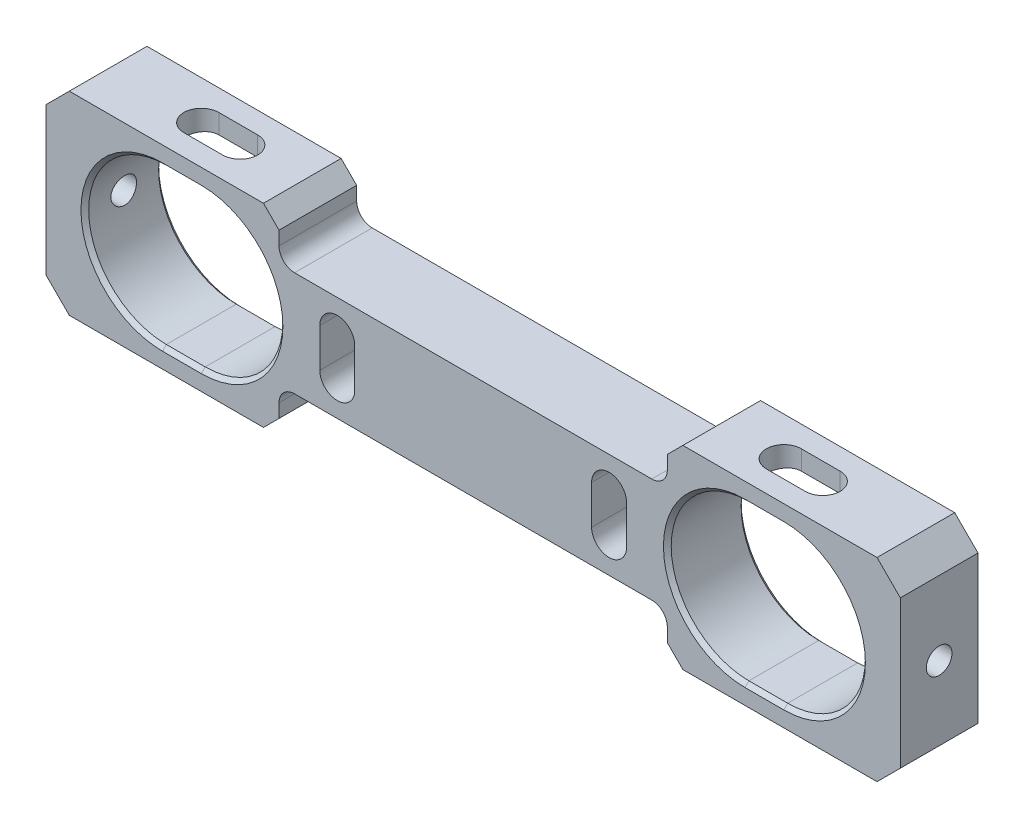
SolidWorks part; units mm, degrees
material "A6061"
ref_plane "Front Plane" through (0, 0, 0) normal (0, 0, 1) x (1, 0, 0)
ref_plane "Top Plane" through (0, 0, 0) normal (0, 1, 0) x (1, 0, 0)
ref_plane "Right Plane" through (0, 0, 0) normal (1, 0, 0) x (0, 0, -1)
sketch "Sketch1" plane through (0, 0, 0) normal (0, 0, 1) x (1, 0, 0)
  line L1 (-55, -12.5) -> (55, -12.5)
  line L2 (-55, -12.5) -> (-55, 12.5)
  line L3 (-55, 12.5) -> (55, 12.5)
  line L4 (55, -12.5) -> (55, 12.5)
  line L5 (-55, -12.5) -> (55, 12.5) construction
  line L6 (-55, 12.5) -> (55, -12.5) construction
  point P0 (0, 0)
  dimension "D1" = 25
  dimension "D2" = 110
extrude "Boss-Extrude1" add sketch "Sketch1" along normal mid plane 10
sketch "Sketch2" plane through (0, 0, 5) normal (0, 0, 1) x (1, 0, 0)
  line L0 (0, 0) -> (0, -23.2819) construction
  line L1 (35, 0) -> (40, 0) construction
  line L2 (35, 10) -> (40, 10)
  line L3 (35, -10) -> (40, -10)
  line L4 (-40, 0) -> (-35, 0) construction
  line L5 (-40, 10) -> (-35, 10)
  line L6 (-40, -10) -> (-35, -10)
  arc A0 (35, 10) -> (35, -10) centre (35, 0) ccw
  arc A1 (40, -10) -> (40, 10) centre (40, 0) ccw
  arc A2 (-40, 10) -> (-40, -10) centre (-40, 0) ccw
  arc A3 (-35, -10) -> (-35, 10) centre (-35, 0) ccw
  point P2 (37.5, 0)
  point P10 (-37.5, 0)
  dimension "D1" = 75
  dimension "D2" = 5
  dimension "D3" = 10
extrude "Cut-Extrude1" cut sketch "Sketch2" against normal through all
chamfer "Chamfer1" distance 3 angle 45 4 edges at (-55, 12.5, 0) (-55, -12.5, 0) (55, -12.5, 0) (55, 12.5, 0)
chamfer "Chamfer2" distance 0.5 angle 45 16 edges at (-50, 0, -5) (-37.5, -10, -5) (-37.5, 10, -5) (-25, 0, -5) (50, 0, -5) (37.5, 10, -5) (37.5, -10, -5) (25, 0, -5) (50, 0, 5) (37.5, 10, 5) (37.5, -10, 5) (25, 0, 5) (-50, 0, 5) (-37.5, -10, 5) (-37.5, 10, 5) (-25, 0, 5)
sketch "Sketch3" plane through (0, 0, 5) normal (0, 0, 1) x (1, 0, 0)
  line L0 (17.5, 2.5) -> (17.5, -2.5) construction
  line L1 (19.75, 2.5) -> (19.75, -2.5)
  line L2 (15.25, 2.5) -> (15.25, -2.5)
  line L3 (-17.5, 2.5) -> (-17.5, -2.5) construction
  line L4 (-15.25, 2.5) -> (-15.25, -2.5)
  line L5 (-19.75, 2.5) -> (-19.75, -2.5)
  line L6 (0, 0) -> (0, -19.6598) construction
  arc A0 (19.75, 2.5) -> (15.25, 2.5) centre (17.5, 2.5) ccw
  arc A1 (15.25, -2.5) -> (19.75, -2.5) centre (17.5, -2.5) ccw
  arc A2 (-15.25, 2.5) -> (-19.75, 2.5) centre (-17.5, 2.5) ccw
  arc A3 (-19.75, -2.5) -> (-15.25, -2.5) centre (-17.5, -2.5) ccw
  point P3 (17.5, 0)
  point P8 (-17.5, 0)
  dimension "D1" = 5
  dimension "D3" = 2.25
  dimension "D2" = 35
extrude "Cut-Extrude2" cut sketch "Sketch3" against normal through all
sketch "Sketch6" plane through (0, 12.5, 0) normal (0, 1, 0) x (1, 0, 0)
  line L0 (-40, 0) -> (-35, 0) construction
  line L1 (-40, 2.25) -> (-35, 2.25)
  line L2 (-40, -2.25) -> (-35, -2.25)
  line L3 (35, 0) -> (40, 0) construction
  line L4 (35, 2.25) -> (40, 2.25)
  line L5 (35, -2.25) -> (40, -2.25)
  line L6 (0, 0) -> (0, -23.5946) construction
  line L7 (-55, -5) -> (-55, 5) construction
  arc A0 (-40, 2.25) -> (-40, -2.25) centre (-40, 0) ccw
  arc A1 (-35, -2.25) -> (-35, 2.25) centre (-35, 0) ccw
  arc A2 (35, 2.25) -> (35, -2.25) centre (35, 0) ccw
  arc A3 (40, -2.25) -> (40, 2.25) centre (40, 0) ccw
  point P3 (-37.5, 0)
  point P8 (37.5, 0)
  dimension "D3" = 2.25
  dimension "D1" = 17.5
  dimension "D2" = 5
extrude "Cut-Extrude3" cut sketch "Sketch6" against normal up to next contours A1 L1 A0 L2
hole_wizard "M4 Tapped Hole1" positions "Sketch8" profile "Sketch7" tap size "M4" standard "ISO"
sketch "Sketch8" plane through (55, 0, 0) normal (1, 0, 0) x (0, 0, -1)
  point P0 (0, 0)
sketch "Sketch7" plane through (55, 0, 0) normal (0, 1, 0) x (0, 0, -1)
  line L0 (0, 0) -> (0, 5)
  line L1 (0, 5) -> (1.65, 5)
  line L2 (1.65, 5) -> (1.65, 0)
  line L5 (1.65, 0) -> (0, 0)
  line L11 (0, -6.35) -> (0, 107.95) construction
  dimension "通孔螺纹孔钻头直径" = 3.3
  dimension "通孔螺纹孔钻头深度" = 5
cosmetic thread "Hole thread1" parameters "D2"=4
hole_wizard "M4 Tapped Hole2" positions "Sketch10" profile "Sketch9" tap size "M4" standard "ISO"
sketch "Sketch10" plane through (-55, 0, 0) normal (-1, 0, 0) x (0, 0, 1)
  point P0 (0, 0)
sketch "Sketch9" plane through (-55, 0, 0) normal (0, 1, 0) x (0, 0, 1)
  line L0 (0, 0) -> (0, 5)
  line L1 (0, 5) -> (1.65, 5)
  line L2 (1.65, 5) -> (1.65, 0)
  line L5 (1.65, 0) -> (0, 0)
  line L11 (0, -6.35) -> (0, 107.95) construction
  dimension "通孔螺纹孔钻头直径" = 3.3
  dimension "通孔螺纹孔钻头深度" = 5
cosmetic thread "Hole thread2" parameters "D2"=4
sketch "Sketch11" plane through (0, 0, -5) normal (0, 0, -1) x (-1, 0, 0)
  line L0 (-17.5, 2.5) -> (-17.5, -2.5) construction
  line L1 (-13.5, 2.5) -> (-13.5, -2.5)
  line L2 (-21.5, 2.5) -> (-21.5, -2.5)
  line L3 (17.5, 2.5) -> (17.5, -2.5) construction
  line L4 (21.5, 2.5) -> (21.5, -2.5)
  line L5 (13.5, 2.5) -> (13.5, -2.5)
  arc A0 (-13.5, 2.5) -> (-21.5, 2.5) centre (-17.5, 2.5) ccw
  arc A1 (-21.5, -2.5) -> (-13.5, -2.5) centre (-17.5, -2.5) ccw
  arc A2 (21.5, 2.5) -> (13.5, 2.5) centre (17.5, 2.5) ccw
  arc A3 (13.5, -2.5) -> (21.5, -2.5) centre (17.5, -2.5) ccw
  point P4 (-17.5, 0)
  point P9 (17.5, 0)
  dimension "D1" = 4
extrude "Cut-Extrude4" cut sketch "Sketch11" against normal blind 4.5
sketch "Sketch12" plane through (0, 0, 5) normal (0, 0, 1) x (1, 0, 0)
  line L0 (-52, -12.5) -> (52, -12.5) construction
  line L1 (-25, -12.5) -> (25, -12.5)
  line L2 (-25, -12.5) -> (-25, -6.75)
  line L3 (-25, -6.75) -> (25, -6.75)
  line L4 (25, -12.5) -> (25, -6.75)
  line L5 (52, 12.5) -> (-52, 12.5) construction
  line L6 (-25, 12.5) -> (25, 12.5)
  line L7 (-25, 12.5) -> (-25, 6.75)
  line L8 (-25, 6.75) -> (25, 6.75)
  line L9 (25, 12.5) -> (25, 6.75)
  line L10 (0, 0) -> (0, -4.6479) construction
  line L11 (0, 0) -> (-8.219, 0) construction
  dimension "D1" = 50
  dimension "D2" = 13.5
extrude "Cut-Extrude5" cut sketch "Sketch12" against normal through all
fillet "Fillet1" radius 2 4 edges at (25, 6.75, 0) (-25, 6.75, 0) (-25, -6.75, 0) (25, -6.75, 0)
chamfer "Chamfer3" distance 2 angle 45 4 edges at (-25, -12.5, 0) (-25, 12.5, 0) (25, -12.5, 0) (25, 12.5, 0)
